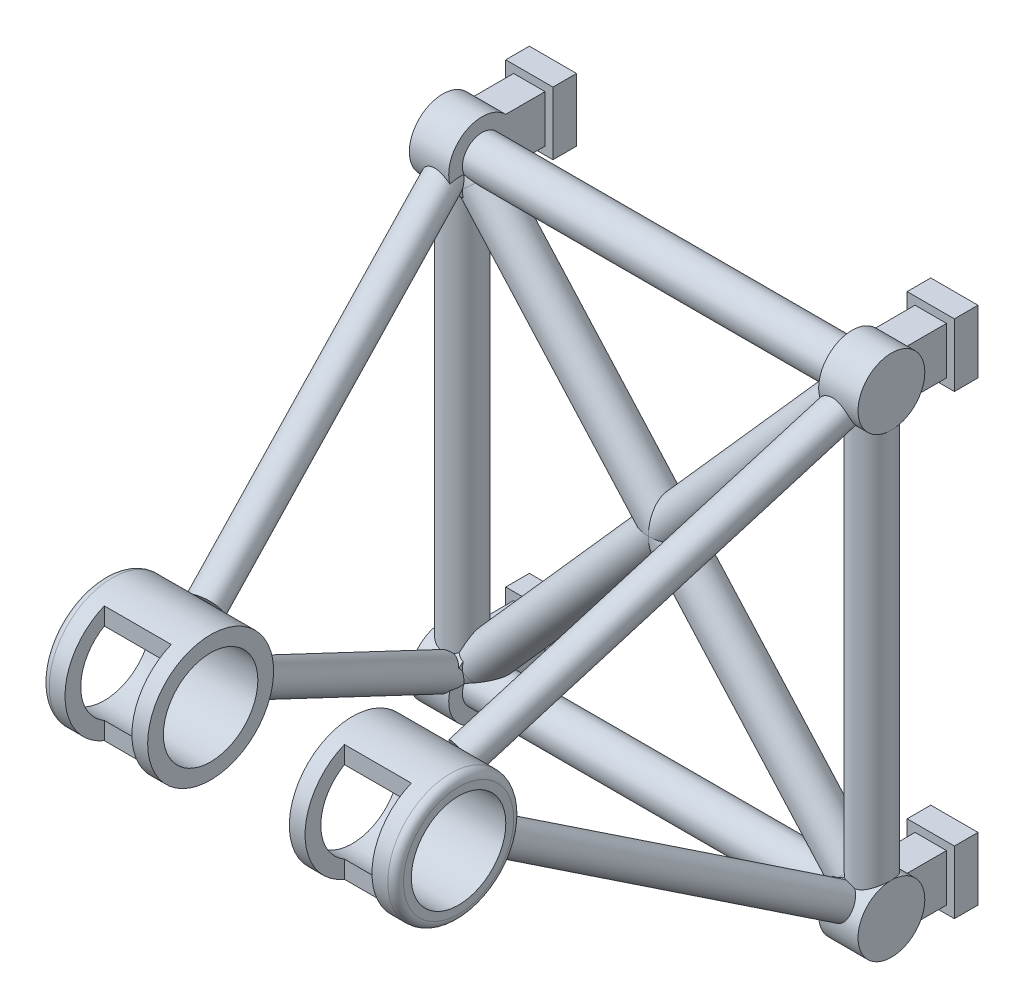
from build123d import *

# Parameters (mm, degrees)
SKETCH1_W                            = 60
SKETCH1_H                            = 80
BOSS_EXTRUDE1_DEPTH                  = 30
BOSS_EXTRUDE1_2_DEPTH                = 30
BOSS_EXTRUDE1_3_DEPTH                = 30
BOSS_EXTRUDE1_4_DEPTH                = 30
SKETCH2_W                            = 40
SKETCH2_H                            = 60
BOSS_EXTRUDE2_DEPTH                  = 50
SKETCH_3_2_R                         = 42.426406871
BOSS_EXTRUDE3_DEPTH                  = 50
BOSS_EXTRUDE4_START                  = 520
SKETCH_3_2_2_R                       = 42.426406871
BOSS_EXTRUDE4_DEPTH                  = 50
BOSS_EXTRUDE5_REACH                  = 465.644
BOSS_EXTRUDE5_END_RADIUS             = 42.426406871
SKETCH4_R                            = 25
BOSS_EXTRUDE5_DIRECTION_2_REACH      = 465.644
BOSS_EXTRUDE5_DIRECTION_2_END_RADIUS = 42.426406871
BOSS_EXTRUDE6_REACH                  = 637.721
SKETCH5_R                            = 25
SWEEP7_PROFILE_R                     = 25
SWEEP8_PROFILE_R                     = 25
SWEEP9_PROFILE_R                     = 20
MIRROR4_COPY_1_SKETCH_R              = 20
SKETCH74_R                           = 80
BOSS_EXTRUDE9_DEPTH                  = 225
FILLET1_R                            = 10
CUT_EXTRUDE1_DEPTH                   = 913.606069063
CUT_EXTRUDE1_DEPTH_BACK              = 913.606069063
SKETCH75_R                           = 60
CUT_EXTRUDE2_DEPTH                   = 809.687107135
CUT_EXTRUDE2_DEPTH_BACK              = 809.687107135
SKETCH76_W                           = 180
SKETCH76_H                           = 160
SKETCH77_W                           = 85
SKETCH77_H                           = 160
CUT_EXTRUDE8_DEPTH                   = 50


with BuildPart() as part:
    # Sketch1 → Boss-Extrude1 (new body)
    with BuildSketch(Plane.XY):
        with Locations((255, 290)):
            Rectangle(SKETCH1_W, SKETCH1_H)
    extrude(amount=BOSS_EXTRUDE1_DEPTH)



with BuildPart() as body_2:
    # Sketch1 → Boss-Extrude1 2 (new body)
    with BuildSketch(Plane.XY):
        with Locations((-255, 290)):
            Rectangle(SKETCH1_W, SKETCH1_H)
    extrude(amount=BOSS_EXTRUDE1_2_DEPTH)


with BuildPart() as body_3:
    # Sketch1 → Boss-Extrude1 3 (new body)
    with BuildSketch(Plane.XY):
        with Locations((-255, -290)):
            Rectangle(SKETCH1_W, SKETCH1_H)
    extrude(amount=BOSS_EXTRUDE1_3_DEPTH)


with BuildPart() as body_4:
    # Sketch1 → Boss-Extrude1 4 (new body)
    with BuildSketch(Plane.XY):
        with Locations((255, -290)):
            Rectangle(SKETCH1_W, SKETCH1_H)
    extrude(amount=BOSS_EXTRUDE1_4_DEPTH)


with BuildPart() as part_1:
    add(part.part)

    add(body_2.part)  # Boss-Extrude2 merges body 2

    add(body_3.part)  # Boss-Extrude2 merges body 3

    add(body_4.part)  # Boss-Extrude2 merges body 4
    # Sketch2 → Boss-Extrude2 (add)
    with BuildSketch(Plane.XY.offset(30)):
        with Locations((-255, -290)):
            Rectangle(SKETCH2_W, SKETCH2_H)
        with Locations((-255, 290)):
            Rectangle(SKETCH2_W, SKETCH2_H)
        with Locations((255, 290)):
            Rectangle(SKETCH2_W, SKETCH2_H)
        with Locations((255, -290)):
            Rectangle(SKETCH2_W, SKETCH2_H)
    extrude(amount=BOSS_EXTRUDE2_DEPTH)

    # Sketch 3_2 → Boss-Extrude3 (add)
    with BuildSketch(Plane(origin=(-235, 0, 0), x_dir=(0, 0, -1), z_dir=(1, 0, 0))):
        with Locations(Location((-110, -290, 0), (0, 0, 90))):
            Circle(SKETCH_3_2_R)
        with Locations(Location((-110, 290, 0), (0, 0, 90))):
            Circle(SKETCH_3_2_R)
    extrude(amount=-BOSS_EXTRUDE3_DEPTH)

    # Sketch 3_2 2 → Boss-Extrude4 (add)
    with BuildSketch(Plane(origin=(-235, 0, 0), x_dir=(0, 0, -1), z_dir=(1, 0, 0)).offset(BOSS_EXTRUDE4_START)):
        with Locations(Location((-110, -290, 0), (0, 0, 315))):
            Circle(SKETCH_3_2_2_R)
        with Locations(Location((-110, 290, 0), (0, 0, 90))):
            Circle(SKETCH_3_2_2_R)
    extrude(amount=-BOSS_EXTRUDE4_DEPTH)

    # Boss-Extrude5: up to this cylinder (the profile starts outside it)
    boss_extrude5_end = Plane(origin=(0, 290, 110), z_dir=(1, 0, 0)) * Cylinder(BOSS_EXTRUDE5_END_RADIUS, 1537.140813742, mode=Mode.PRIVATE)
    # Sketch4 → Boss-Extrude5 (add, up to the surface)
    with BuildSketch(Plane(origin=(0, 0, 0), x_dir=(1, 0, 0), z_dir=(0, 1, 0)), mode=Mode.PRIVATE) as boss_extrude5_sk1:
        with Locations((260, -110)):
            Circle(SKETCH4_R)
    boss_extrude5_tool1 = extrude(boss_extrude5_sk1.sketch, amount=BOSS_EXTRUDE5_REACH, mode=Mode.PRIVATE) - boss_extrude5_end
    add(boss_extrude5_tool1.solids().sort_by_distance((260, 0, 110))[0])
    # Sketch4 → Boss-Extrude5 (add, up to the surface)
    with BuildSketch(Plane(origin=(0, 0, 0), x_dir=(1, 0, 0), z_dir=(0, 1, 0)), mode=Mode.PRIVATE) as boss_extrude5_sk2:
        with Locations(Location((-260, -110, 0), (0, 0, 180))):
            Circle(SKETCH4_R)
    boss_extrude5_tool2 = extrude(boss_extrude5_sk2.sketch, amount=BOSS_EXTRUDE5_REACH, mode=Mode.PRIVATE) - boss_extrude5_end
    add(boss_extrude5_tool2.solids().sort_by_distance((-260, 0, 110))[0])

    # Boss-Extrude5 direction 2: up to this cylinder (the profile starts outside it)
    boss_extrude5_direction_2_end = Plane(origin=(0, -290, 110), z_dir=(1, 0, 0)) * Cylinder(BOSS_EXTRUDE5_DIRECTION_2_END_RADIUS, 1537.140813742, mode=Mode.PRIVATE)
    # Sketch4 → Boss-Extrude5 direction 2 (add, up to the surface)
    with BuildSketch(Plane(origin=(0, 0, 0), x_dir=(1, 0, 0), z_dir=(0, 1, 0)), mode=Mode.PRIVATE) as boss_extrude5_direction_2_sk1:
        with Locations((260, -110)):
            Circle(SKETCH4_R)
    boss_extrude5_direction_2_tool1 = extrude(boss_extrude5_direction_2_sk1.sketch, amount=-BOSS_EXTRUDE5_DIRECTION_2_REACH, mode=Mode.PRIVATE) - boss_extrude5_direction_2_end
    add(boss_extrude5_direction_2_tool1.solids().sort_by_distance((260, 0, 110))[0])
    # Sketch4 → Boss-Extrude5 direction 2 (add, up to the surface)
    with BuildSketch(Plane(origin=(0, 0, 0), x_dir=(1, 0, 0), z_dir=(0, 1, 0)), mode=Mode.PRIVATE) as boss_extrude5_direction_2_sk2:
        with Locations(Location((-260, -110, 0), (0, 0, 180))):
            Circle(SKETCH4_R)
    boss_extrude5_direction_2_tool2 = extrude(boss_extrude5_direction_2_sk2.sketch, amount=-BOSS_EXTRUDE5_DIRECTION_2_REACH, mode=Mode.PRIVATE) - boss_extrude5_direction_2_end
    add(boss_extrude5_direction_2_tool2.solids().sort_by_distance((-260, 0, 110))[0])

    # Sketch5 → Boss-Extrude6 (add, up to next)
    with BuildSketch(Plane(origin=(-235, 0, 0), x_dir=(0, 0, -1), z_dir=(1, 0, 0)), mode=Mode.PRIVATE) as boss_extrude6_sk1:
        with Locations((-110, -290)):
            Circle(SKETCH5_R)
    boss_extrude6_tool1 = extrude(boss_extrude6_sk1.sketch, amount=BOSS_EXTRUDE6_REACH, mode=Mode.PRIVATE) - part_1.part
    # Sketch5 → Boss-Extrude6 (add, up to next)
    with BuildSketch(Plane(origin=(-235, 0, 0), x_dir=(0, 0, -1), z_dir=(1, 0, 0)), mode=Mode.PRIVATE) as boss_extrude6_sk2:
        with Locations(Location((-110, 290, 0), (0, 0, 216.952075835))):
            Circle(SKETCH5_R)
    boss_extrude6_tool2 = extrude(boss_extrude6_sk2.sketch, amount=BOSS_EXTRUDE6_REACH, mode=Mode.PRIVATE) - part_1.part
    add(boss_extrude6_tool1.solids().sort_by_distance((-235, -290, 110))[0])
    add(boss_extrude6_tool2.solids().sort_by_distance((-235, 290, 110))[0])

    # Sweep7: sweep along a path in Sketch6
    with BuildLine(Plane.XY.offset(110)) as sweep7_path:
        Line((251.524376168, 283.633870998), (235, 265))
        Line((235, 265), (-235, -265))
        Line((-235, -265), (-252.569489109, -282.569489109))
    # Sweep7 profile (on start of the path) → Sweep7 (sweep)
    with BuildSketch(Plane(origin=(251.524376168, 283.633870998, 110), x_dir=(-0.7481876601566486, 0.6634871703275952, 0), z_dir=(-0.6634871703275952, -0.7481876601566486, 0))):
        Circle(SWEEP7_PROFILE_R)
    sweep(path=sweep7_path.line, transition=Transition.RIGHT)

    # Sweep8: sweep along a path in Sketch22
    with BuildLine(Plane.XY.offset(110)) as sweep8_path:
        Line((-254.222570049, 286.472019736), (-235, 265))
        Line((-235, 265), (235, -260))
        Line((235, -260), (256.263290564, -283.75154797))
    # Sweep8 profile (on start of the path) → Sweep8 (sweep)
    with BuildSketch(Plane(origin=(-254.222570049, 286.472019736, 110), x_dir=(-0.7450557030210551, -0.6670022484188503, 0), z_dir=(0.6670022484188503, -0.7450557030210551, 0))):
        Circle(SWEEP8_PROFILE_R)
    sweep(path=sweep8_path.line)

    # Sweep9: sweep along a curve in space
    with BuildLine() as sweep9_path:
        Line((-260, 290, 110), (-164.339575112, 40, 532.313962722))
    # Sweep9 profile (on start of the path) → Sweep9 (sweep)
    with BuildSketch(Plane(origin=(-260, 290, 110), x_dir=(0, 0.8605239098916388, 0.5094100514367642), z_dir=(0.19132084977502523, -0.49999999999999706, 0.8446279254449057))):
        Circle(SWEEP9_PROFILE_R)
    sweep9 = sweep(path=sweep9_path.line)

    # Mirror3: Sweep9 across plane
    add(sweep9.mirror(Plane(origin=(0, 0, 0), x_dir=(0, 0, 1), z_dir=(1, 0, 0))))

    # Mirror4: Sweep9 across plane
    add(sweep9.mirror(Plane.ZX))

    # Mirror4 copy 1: sweep along a curve in space
    with BuildLine() as mirror4_copy_1_path:
        Line((260, -290, 110), (164.339575112, -40, 532.313962722))
    # Mirror4 copy 1 sketch → Mirror4 copy 1 (sweep)
    with BuildSketch(Plane(origin=(260, -290, 110), x_dir=(0, -0.8605239098916388, 0.5094100514367642), z_dir=(-0.19132084977502523, 0.49999999999999706, 0.8446279254449057))):
        Circle(MIRROR4_COPY_1_SKETCH_R)
    sweep(path=mirror4_copy_1_path.line)

    # Sketch74 → Boss-Extrude9 (add, symmetric)
    with BuildSketch(Plane(origin=(0, 0, 0), x_dir=(0, 0, -1), z_dir=(1, 0, 0))):
        with Locations((-599.884196758, 0)):
            Circle(SKETCH74_R)
    extrude(amount=BOSS_EXTRUDE9_DEPTH, both=True)

    # Fillet1
    fillet1_edges = [part_1.edges().sort_by_distance(p)[0] for p in [
        (-225, 0, 679.884196758),
        (225, 0, 679.884196758),
    ]]
    fillet(fillet1_edges, radius=FILLET1_R)

    # Sketch75 → Cut-Extrude1 (cut, two sides: drawn at the far end of the back side and taken through both)
    with BuildSketch(Plane(origin=(225, 0, 0), x_dir=(0, 0, -1), z_dir=(1, 0, 0)).offset(-CUT_EXTRUDE1_DEPTH_BACK)):
        with Locations((-599.884196758, 0)):
            Circle(SKETCH75_R)
    extrude(amount=CUT_EXTRUDE1_DEPTH + CUT_EXTRUDE1_DEPTH_BACK, mode=Mode.SUBTRACT)

    # Sketch76 → Cut-Extrude2 (cut, two sides: drawn at the far end of the back side and taken through both)
    with BuildSketch(Plane(origin=(0, 0, 0), x_dir=(1, 0, 0), z_dir=(0, 1, 0)).offset(-CUT_EXTRUDE2_DEPTH_BACK)):
        with Locations((0, -599.884196758)):
            Rectangle(SKETCH76_W, SKETCH76_H)
    extrude(amount=CUT_EXTRUDE2_DEPTH + CUT_EXTRUDE2_DEPTH_BACK, mode=Mode.SUBTRACT)

    # Sketch77 → Cut-Extrude8 (cut)
    with BuildSketch(Plane.XY.offset(679.884196758)):
        with Locations((152.5, 0)):
            Rectangle(SKETCH77_W, SKETCH77_H)
        with Locations((-152.5, 0)):
            Rectangle(SKETCH77_W, SKETCH77_H)
    extrude(amount=-CUT_EXTRUDE8_DEPTH, mode=Mode.SUBTRACT)


solid = part_1.part
